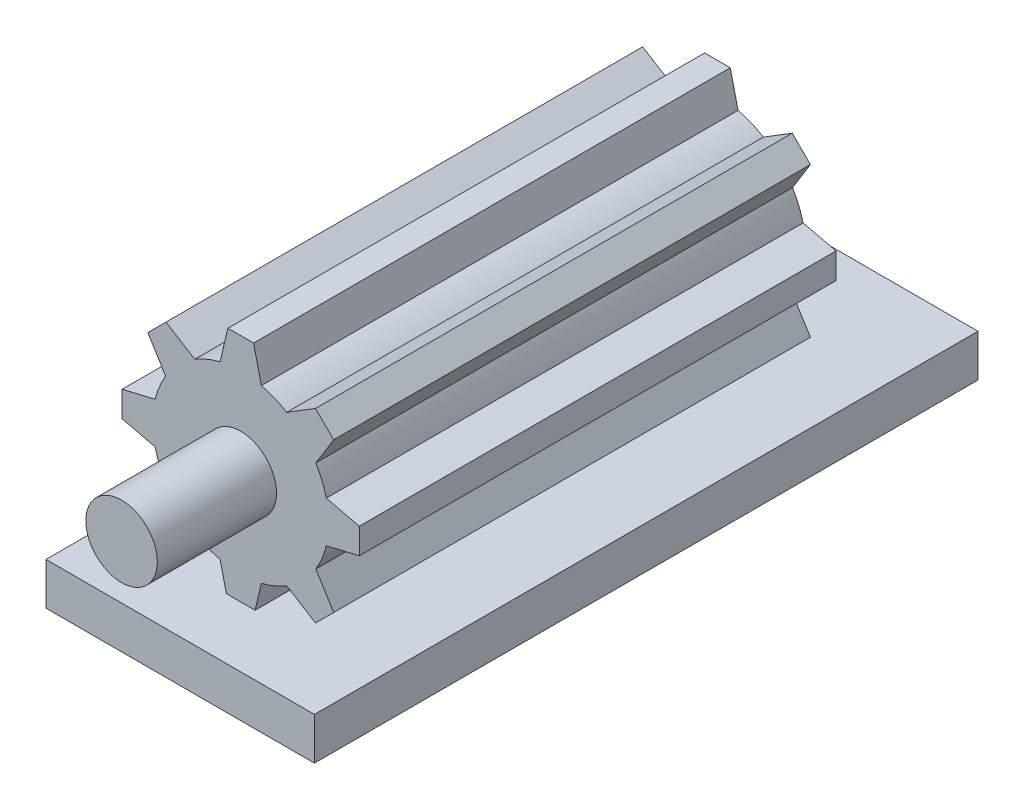
SolidWorks part; units mm, degrees
ref_plane "Front Plane" through (0, 0, 0) normal (0, 0, 1) x (1, 0, 0)
ref_plane "Top Plane" through (0, 0, 0) normal (0, 1, 0) x (1, 0, 0)
ref_plane "Right Plane" through (0, 0, 0) normal (1, 0, 0) x (0, 0, -1)
sketch "Sketch1" plane through (0, 0, 0) normal (0, 0, 1) x (1, 0, 0)
  circle A0 centre (0, 0) radius 150
  dimension "D1" = 300
extrude "Boss-Extrude1" add sketch "Sketch1" against normal blind 3000
sketch "Sketch2" plane through (0, 0, 0) normal (0, 1, 0) x (1, 0, 0)
  line L0 (0, 150) -> (0, 450) construction
  line L1 (-50, 150) -> (-50, 450)
  line L2 (50, 150) -> (50, 450)
  arc A0 (-50, 150) -> (50, 150) centre (0, 150) ccw
  arc A1 (50, 450) -> (-50, 450) centre (0, 450) ccw
  point P3 (0, 300)
  dimension "D2" = 50
  dimension "D1" = 300
  dimension "D3" = 150
extrude "Cut-Extrude1" cut sketch "Sketch2" along normal blind 435
sketch "Sketch4" plane through (0, 0, -3000) normal (0, 0, -1) x (-1, 0, 0)
  line L0 (-86.4993, 359.1162) -> (-53.8465, 497.4777)
  line L1 (0, 600.3487) -> (0, 497.4777) construction
  line L2 (-53.8465, 497.4777) -> (53.8465, 497.4777)
  line L3 (86.4993, 359.1162) -> (53.8465, 497.4777)
  line L4 (192.7693, 315.0977) -> (313.6946, 389.8451)
  line L5 (313.6946, 389.8451) -> (389.8451, 313.6946)
  line L6 (315.0977, 192.7693) -> (389.8451, 313.6946)
  line L7 (359.1162, 86.4993) -> (497.4777, 53.8465)
  line L8 (497.4777, 53.8465) -> (497.4777, -53.8465)
  line L9 (359.1162, -86.4993) -> (497.4777, -53.8465)
  line L10 (315.0977, -192.7693) -> (389.8451, -313.6946)
  line L11 (389.8451, -313.6946) -> (313.6946, -389.8451)
  line L12 (192.7693, -315.0977) -> (313.6946, -389.8451)
  line L13 (86.4993, -359.1162) -> (53.8465, -497.4777)
  line L14 (53.8465, -497.4777) -> (-53.8465, -497.4777)
  line L15 (-86.4993, -359.1162) -> (-53.8465, -497.4777)
  line L16 (-192.7693, -315.0977) -> (-313.6946, -389.8451)
  line L17 (-313.6946, -389.8451) -> (-389.8451, -313.6946)
  line L18 (-315.0977, -192.7693) -> (-389.8451, -313.6946)
  line L19 (-359.1162, -86.4993) -> (-497.4777, -53.8465)
  line L20 (-497.4777, -53.8465) -> (-497.4777, 53.8465)
  line L21 (-359.1162, 86.4993) -> (-497.4777, 53.8465)
  line L22 (-315.0977, 192.7693) -> (-389.8451, 313.6946)
  line L23 (-389.8451, 313.6946) -> (-313.6946, 389.8451)
  line L24 (-192.7693, 315.0977) -> (-313.6946, 389.8451)
  arc A0 (-86.4993, 359.1162) -> (-192.7693, 315.0977) centre (0, 0) ccw
  arc A1 (-315.0977, 192.7693) -> (-359.1162, 86.4993) centre (0, 0) ccw
  arc A2 (-359.1162, -86.4993) -> (-315.0977, -192.7693) centre (0, 0) ccw
  arc A3 (-192.7693, -315.0977) -> (-86.4993, -359.1162) centre (0, 0) ccw
  arc A4 (86.4993, -359.1162) -> (192.7693, -315.0977) centre (0, 0) ccw
  arc A5 (315.0977, -192.7693) -> (359.1162, -86.4993) centre (0, 0) ccw
  arc A6 (359.1162, 86.4993) -> (315.0977, 192.7693) centre (0, 0) ccw
  arc A7 (192.7693, 315.0977) -> (86.4993, 359.1162) centre (0, 0) ccw
  point P9 (0, 497.4777)
  point P17 (351.7699, 351.7699)
  point P22 (497.4777, 0)
  point P27 (351.7699, -351.7699)
  point P32 (0, -497.4777)
  point P37 (-351.7699, -351.7699)
  point P42 (-497.4777, 0)
  point P47 (-351.7699, 351.7699)
  point P48 (0, 0)
  dimension "D1" = 8
extrude "Boss-Extrude3" add sketch "Sketch4" along normal blind 2000
sketch "Sketch5" plane through (0, 0, -5000) normal (0, 0, -1) x (-1, 0, 0)
  line L1 (-563.0289, -647.4043) -> (563.0289, -647.4043)
  line L2 (-563.0289, -647.4043) -> (-563.0289, -470.229)
  line L3 (-563.0289, -470.229) -> (563.0289, -470.229)
  line L4 (563.0289, -647.4043) -> (563.0289, -470.229)
  line L5 (-563.0289, -647.4043) -> (563.0289, -470.229) construction
  line L6 (-563.0289, -470.229) -> (563.0289, -647.4043) construction
  point P0 (0, -558.8167)
extrude "Boss-Extrude4" add sketch "Sketch5" against normal blind 2254 and the other way blind 530
sketch "Sketch6" plane through (0, 0, 0) normal (0, 1, 0) x (1, 0, 0)
  line L2 (50, 150) -> (50, 450)
  line L3 (-50, 450) -> (-50, 150)
  line L4 (50, 150) -> (50, 450)
  line L5 (-50, 450) -> (-50, 150)
  arc A2 (-50, 150) -> (50, 150) centre (0, 150) ccw
  arc A3 (50, 450) -> (-50, 450) centre (0, 450) ccw
  arc A4 (-50, 150) -> (50, 150) centre (0, 150) ccw
  arc A5 (50, 450) -> (-50, 450) centre (0, 450) ccw
  dimension "D1" = 0
extrude "Boss-Extrude5" add sketch "Sketch6" along normal blind 75
sketch "Sketch8" plane through (0, 0, 0) normal (0, 0, 1) x (1, 0, 0)
  circle A0 centre (0, 0) radius 377.2536
extrude "Cut-Extrude2" cut sketch "Sketch8" against normal blind 2500
